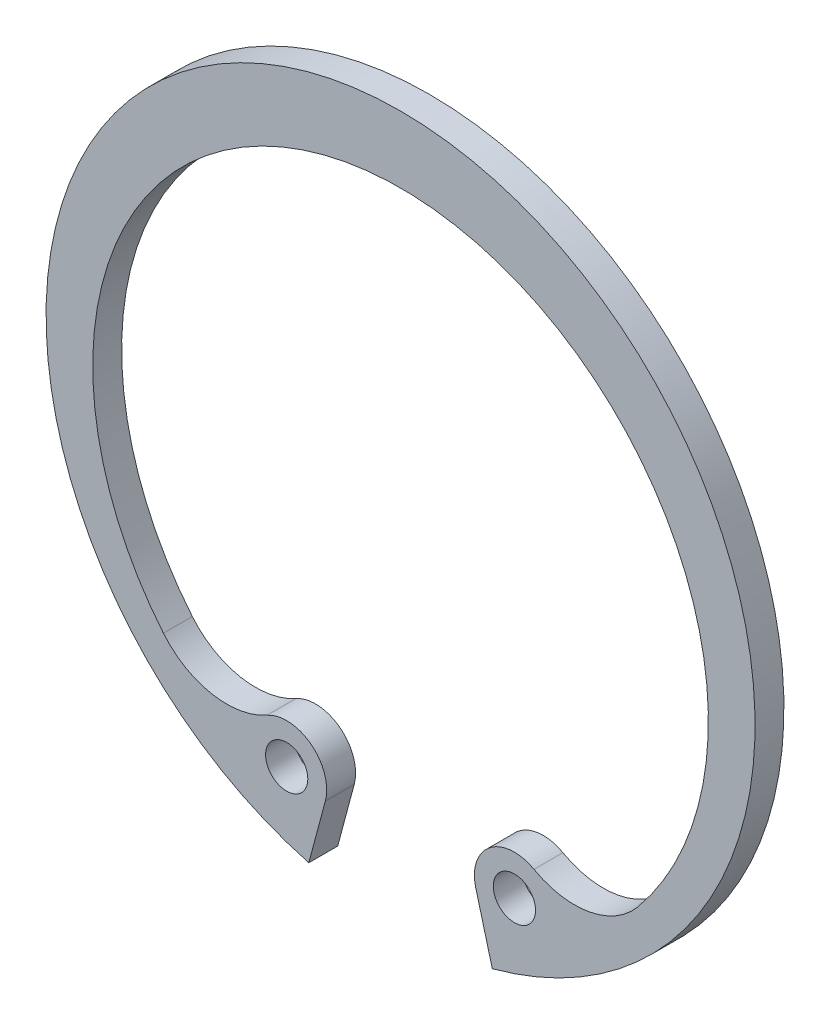
SolidWorks part; units mm, degrees
ref_plane "Front Plane" through (0, 0, 0) normal (0, 0, 1) x (1, 0, 0)
ref_plane "Top Plane" through (0, 0, 0) normal (0, 1, 0) x (1, 0, 0)
ref_plane "Right Plane" through (0, 0, 0) normal (1, 0, 0) x (0, 0, -1)
sketch "Sketch1" plane through (0, 0, 0) normal (0, 0, 1) x (1, 0, 0)
  line L0 (0, 0) -> (0, 0.9) construction
  line L1 (0, 0.9) -> (3.3845, -11.7311) construction
  line L2 (0, 0.9) -> (-3.3845, -11.7311) construction
  line L3 (3.3845, -11.7311) -> (4.1282, -14.5065)
  line L4 (-3.3845, -11.7311) -> (-4.1282, -14.5065)
  arc A4 (10.6698, -8.8305) -> (-10.6698, -8.8305) centre (0, 0) ccw
  arc A5 (4.1282, -14.5065) -> (-4.1282, -14.5065) centre (0, 0.9) ccw
  circle A6 centre (5.1232, -11.2652) radius 0.95
  arc A7 (6.0056, -9.6964) -> (10.6698, -8.8305) centre (7.8194, -6.4715) ccw
  arc A8 (6.0056, -9.6964) -> (3.3845, -11.7311) centre (5.1232, -11.2652) ccw
  arc A9 (-6.0056, -9.6964) -> (-3.3845, -11.7311) centre (-5.1232, -11.2652) cw
  arc A10 (-6.0056, -9.6964) -> (-10.6698, -8.8305) centre (-7.8194, -6.4715) cw
  circle A11 centre (-5.1232, -11.2652) radius 0.95
  arc A12 (-10.6698, -8.8305) -> (10.6698, -8.8305) centre (0, 0) cw
  dimension "D1" = 27.7
  dimension "D3" = 31.9
  dimension "D2" = 0.9
  dimension "D4" = 13.2
  dimension "D5" = 3.7
  dimension "D7" = 3.6
  dimension "D8" = 1.9
  dimension "D6" = 15
extrude "Boss-Extrude1" add sketch "Sketch1" along normal blind 1.3 contours A9 A10 A4 A7 A8 L3 A5 L4 A6 A11
